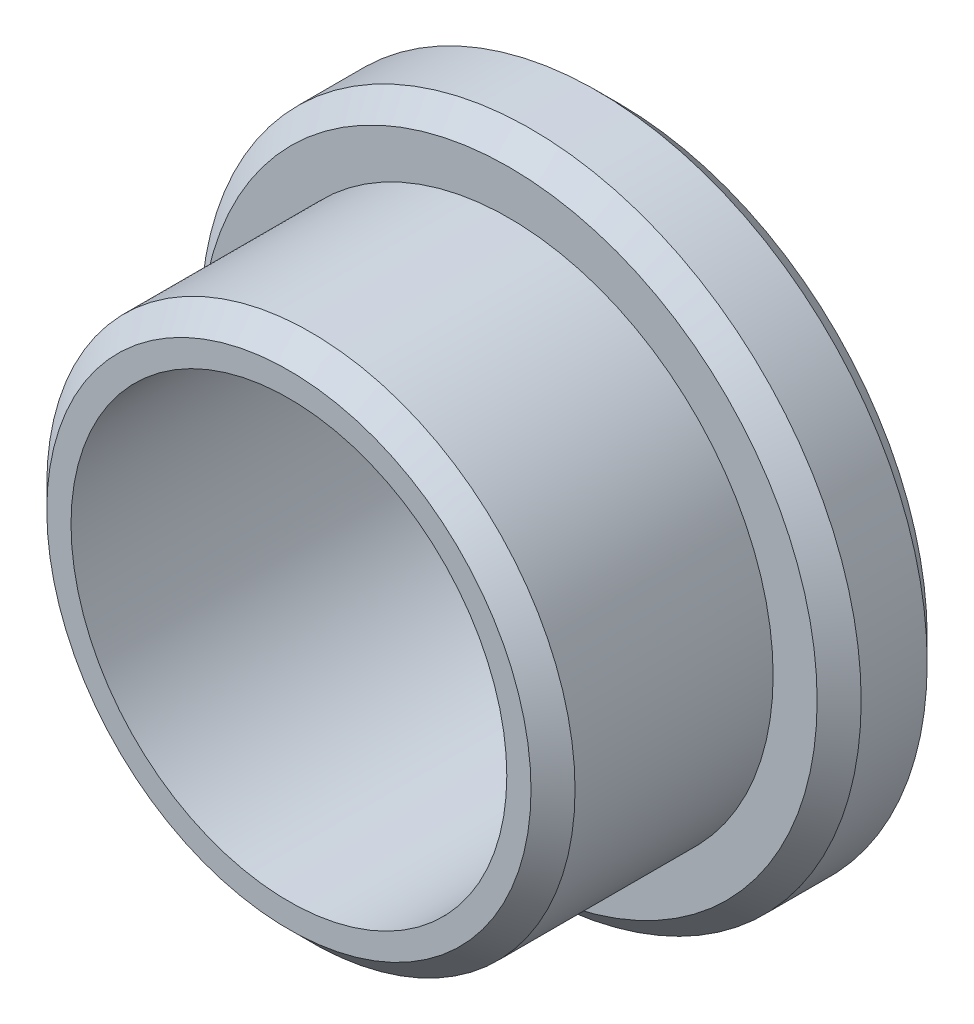
from build123d import *

# Parameters (mm, degrees)
SKETCH2_R           = 15
SKETCH2_R_2         = 9.9
BOSS_EXTRUDE1_DEPTH = 5
SKETCH3_R           = 12
SKETCH3_R_2         = 9.9
BOSS_EXTRUDE2_DEPTH = 10
CHAMFER1_SIZE       = 1


with BuildPart() as part:
    # Sketch2 → Boss-Extrude1 (new body)
    with BuildSketch(Plane.XY):
        Circle(SKETCH2_R)
        Circle(SKETCH2_R_2, mode=Mode.SUBTRACT)
    extrude(amount=BOSS_EXTRUDE1_DEPTH)

    # Sketch3 → Boss-Extrude2 (add)
    with BuildSketch(Plane.XY.offset(5)):
        Circle(SKETCH3_R)
        Circle(SKETCH3_R_2, mode=Mode.SUBTRACT)
    extrude(amount=BOSS_EXTRUDE2_DEPTH)

    # Chamfer1
    chamfer1_edges = [part.edges().sort_by_distance(p)[0] for p in [
        (-12, 0, 15),
        (-15, 0, 0),
        (-15, 0, 5),
    ]]
    chamfer(chamfer1_edges, length=CHAMFER1_SIZE)


solid = part.part
